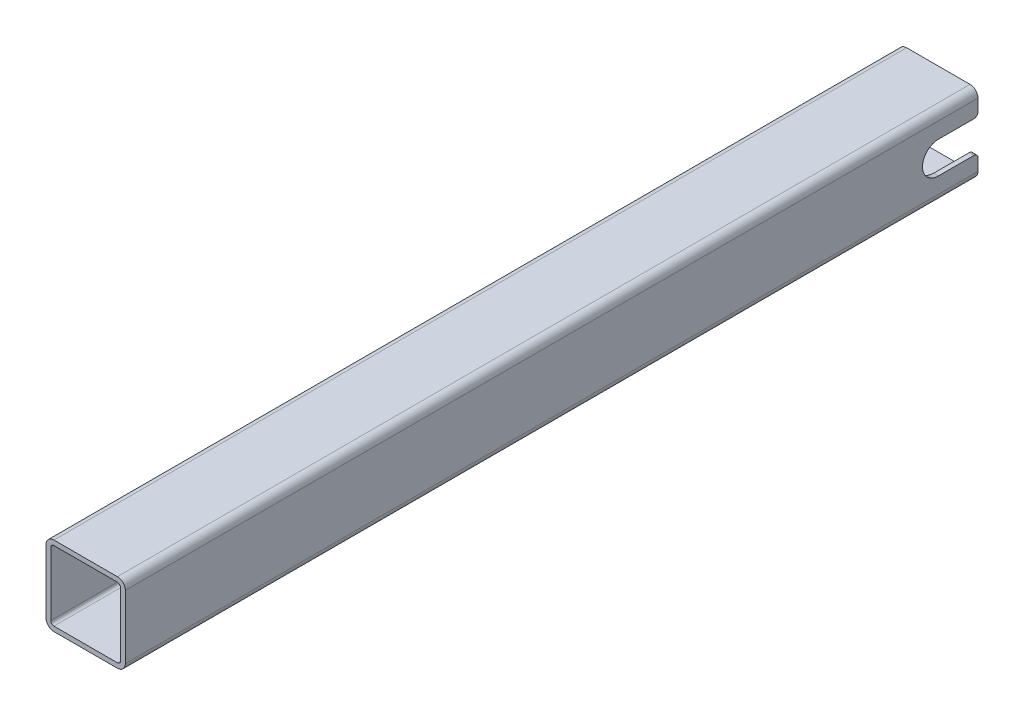
SolidWorks part; units mm, degrees
material "QT800-2"
ref_plane "前视基准面" through (0, 0, 0) normal (0, 0, 1) x (1, 0, 0)
ref_plane "上视基准面" through (0, 0, 0) normal (0, 1, 0) x (1, 0, 0)
ref_plane "右视基准面" through (0, 0, 0) normal (1, 0, 0) x (0, 0, -1)
sketch "草图1" plane through (0, 0, 0) normal (0, 0, 1) x (1, 0, 0)
  line L0 (-80, 88) -> (80, 88)
  line L1 (-80, 100) -> (80, 100)
  line L2 (-100, 80) -> (-100, -80)
  line L3 (-80, -100) -> (80, -100)
  line L4 (100, 80) -> (100, -80)
  line L5 (-100, 100) -> (100, -100) construction
  line L6 (-100, -100) -> (100, 100) construction
  line L7 (88, 80) -> (88, -80)
  line L8 (-80, -88) -> (80, -88)
  line L9 (-88, 80) -> (-88, -80)
  arc A0 (80, -100) -> (100, -80) centre (80, -80) ccw
  arc A1 (-80, -100) -> (-100, -80) centre (-80, -80) cw
  arc A2 (100, 80) -> (80, 100) centre (80, 80) ccw
  arc A3 (-100, 80) -> (-80, 100) centre (-80, 80) cw
  arc A4 (88, 80) -> (80, 88) centre (80, 80) ccw
  arc A5 (80, -88) -> (88, -80) centre (80, -80) ccw
  arc A6 (-80, -88) -> (-88, -80) centre (-80, -80) cw
  arc A7 (-88, 80) -> (-80, 88) centre (-80, 80) cw
  point P0 (0, 0)
  dimension "D3" = 20
  dimension "D1" = 200
  dimension "D2" = 200
  dimension "D4" = 12
extrude "凸台-拉伸1" add sketch "草图1" along normal blind 2150
sketch "草图3" plane through (100, 0, 0) normal (1, 0, 0) x (0, 0, -1)
  line L0 (-100, 0) -> (100, 0) construction
  line L1 (-100, 40) -> (100, 40)
  line L2 (-100, -40) -> (100, -40)
  line L3 (0, -80) -> (0, 80) construction
  arc A0 (-100, 40) -> (-100, -40) centre (-100, 0) ccw
  arc A1 (100, -40) -> (100, 40) centre (100, 0) ccw
  point P2 (0, 0)
  dimension "D1" = 40
  dimension "D2" = 100
extrude "切除-拉伸2" cut sketch "草图3" against normal up to surface (12 mm away) up to face at (88, 0, 1075)
fillet "圆角1" radius 10 2 edges at (94, -40, 0) (94, 40, 0)
